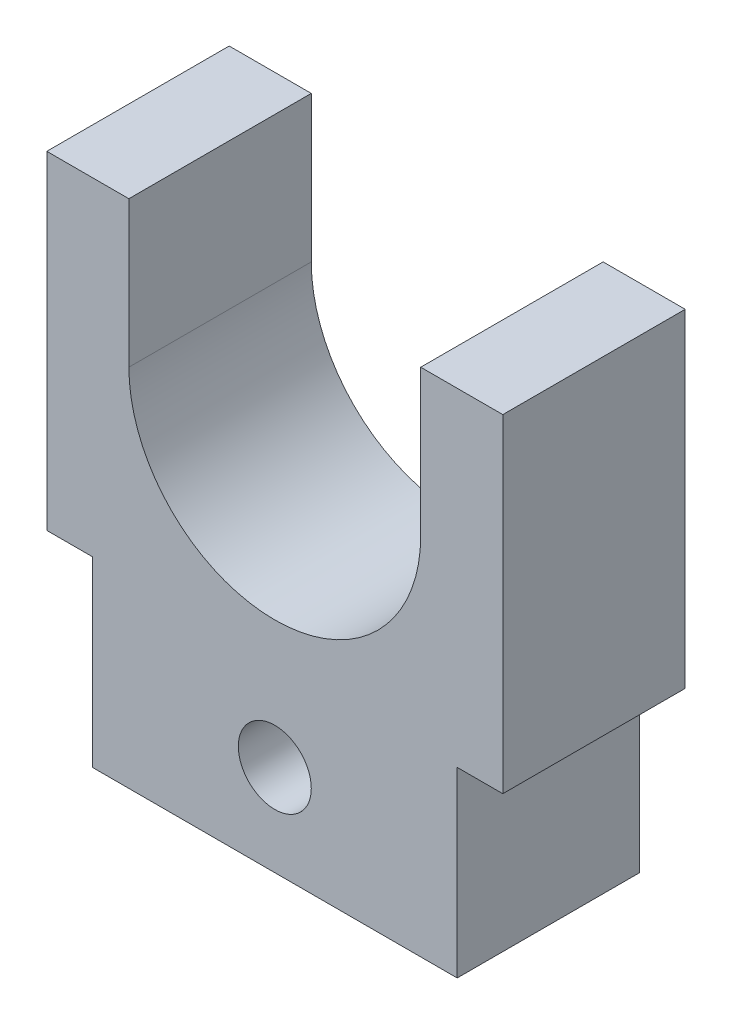
from build123d import *

# Parameters (mm, degrees)
SKETCH_1_R      = 2
EXTRUDE_1_DEPTH = 10


with BuildPart() as part:
    # 草图1 → 凸台-拉伸1 (new body)
    with BuildSketch(Plane.XY):
        with BuildLine():
            Line((0, 10), (-2.5, 10))
            Line((-2.5, 10), (-2.5, 27.142110135))
            Line((-2.5, 27.142110135), (-2.5, 28))
            Line((-2.5, 28), (2, 28))
            Line((2, 28), (2, 20))
            ThreePointArc((2, 20), (10, 12), (18, 20))
            Line((18, 20), (18, 28))
            Line((18, 28), (22.5, 28))
            Line((22.5, 28), (22.5, 10))
            Line((22.5, 10), (20, 10))
            Line((20, 10), (20, 0))
            Line((20, 0), (0, 0))
            Line((0, 0), (0, 10))
        make_face()
        with Locations((10, 5)):
            Circle(SKETCH_1_R, mode=Mode.SUBTRACT)
    extrude(amount=EXTRUDE_1_DEPTH)


solid = part.part
